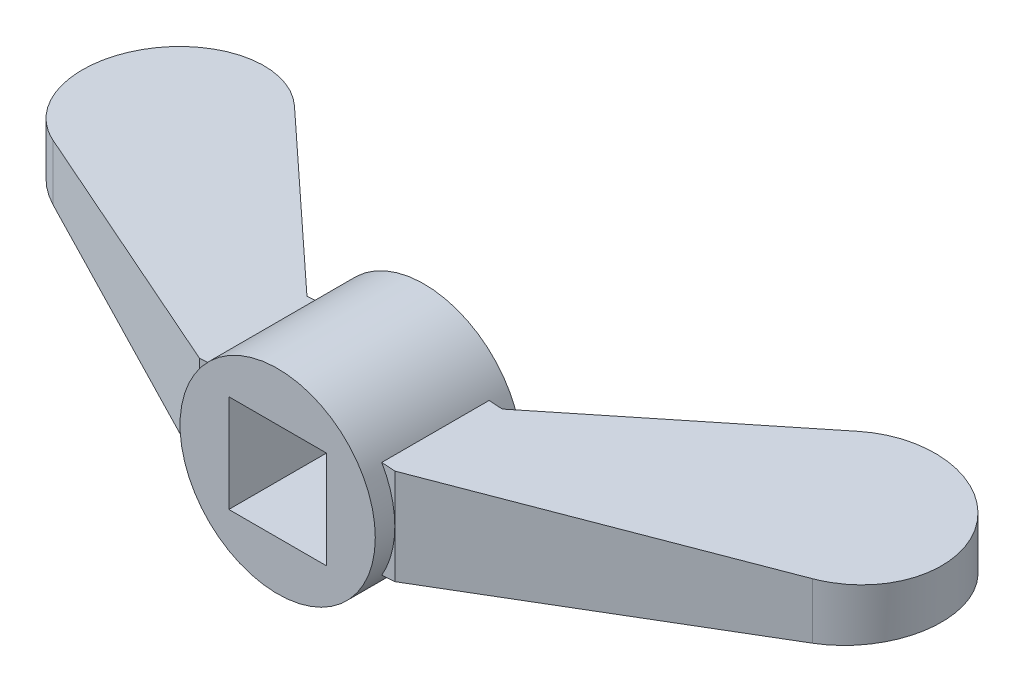
SolidWorks part; units mm, degrees
ref_plane "Front Plane" through (0, 0, 0) normal (0, 0, 1) x (1, 0, 0)
ref_plane "Top Plane" through (0, 0, 0) normal (0, 1, 0) x (1, 0, 0)
ref_plane "Right Plane" through (0, 0, 0) normal (1, 0, 0) x (0, 0, -1)
sketch "Sketch1" plane through (0, 0, 0) normal (0, 0, 1) x (1, 0, 0)
  line L1 (-5, -5) -> (5, -5)
  line L2 (-5, -5) -> (-5, 5)
  line L3 (-5, 5) -> (5, 5)
  line L4 (5, -5) -> (5, 5)
  line L5 (-5, -5) -> (5, 5) construction
  line L6 (-5, 5) -> (5, -5) construction
  circle A0 centre (0, 0) radius 10
  dimension "D1" = 20
  dimension "D2" = 10
  dimension "D3" = 10
extrude "Boss-Extrude1" add sketch "Sketch1" along normal mid plane 15
sketch "Sketch2" plane through (0, 0, 0) normal (0, 1, 0) x (1, 0, 0)
  line L0 (-10, -7.5) -> (10, -7.5) construction
  line L1 (-28.8633, 23.0834) -> (-10, 5.5)
  line L2 (-10, 7.5) -> (-10, -7.5) construction
  line L3 (10, 7.5) -> (-10, 7.5) construction
  line L4 (-38.8984, 8.3881) -> (-10, -5.5)
  line L5 (-10, 5.5) -> (-8, 5.5)
  line L6 (-8, 5.5) -> (-8, -5.5)
  line L7 (-8, -5.5) -> (-10, -5.5)
  circle A0 centre (-35, 16.5) radius 9
  dimension "D1" = 18
  dimension "D2" = 35
  dimension "D3" = 24
  dimension "D4" = 2
  dimension "D5" = 2
  dimension "D6" = 2
extrude "Boss-Extrude2" add sketch "Sketch2" along normal mid plane 10 contours A0 | A0 L4 L7 L6 L5 L1
sketch "Sketch3" plane through (0, 0, 0) normal (0, 0, 1) x (1, 0, 0)
  line L0 (-8.6603, 5) -> (-44, 2.5)
  line L1 (-44, 5) -> (-44, -5) construction
  line L2 (-44, -2.5) -> (-8.6603, -5)
  line L3 (-44, 2.5) -> (-51.2929, 13.0405)
  line L4 (-51.2929, 13.0405) -> (-8.6603, 5)
  line L5 (-44, -2.5) -> (-51.2929, -11.4451)
  line L6 (-51.2929, -11.4451) -> (-8.6603, -5)
  line L7 (-8.6603, -5) -> (-8.8721, -4.8948)
  dimension "D1" = 2.5
  dimension "D2" = 2.5
extrude "Cut-Extrude1" cut sketch "Sketch3" against normal mid plane 76 contours L4 L3 L0 | L5 L6 L2
mirror "Mirror1" about plane through (0, 0, 0) normal (1, 0, 0) of "Boss-Extrude2", "Cut-Extrude1"
